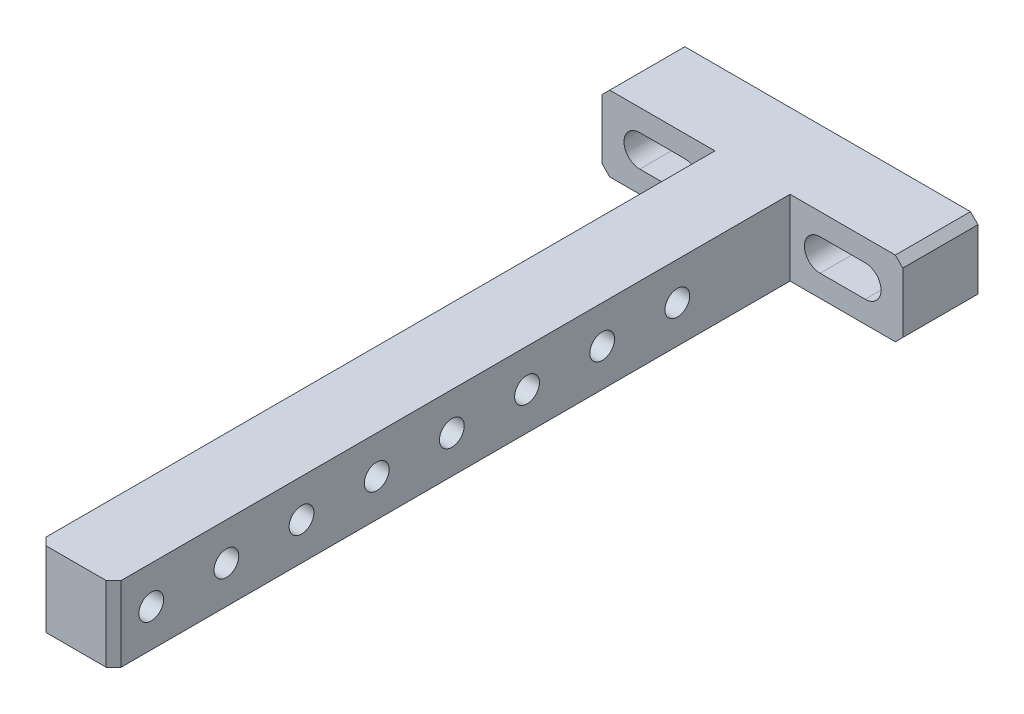
from build123d import *

# Parameters (mm, degrees)
SKETCH1_W           = 40
SKETCH1_H           = 10
BOSS_EXTRUDE1_DEPTH = 10
SKETCH2_W           = 10
SKETCH2_H           = 10
BOSS_EXTRUDE2_DEPTH = 90
CUT_EXTRUDE1_DEPTH  = 103.102889283
M4_TAPPED_HOLE1_D   = 3.3
CHAMFER1_SIZE       = 1


with BuildPart() as part:
    # Sketch1 → Boss-Extrude1 (new body)
    with BuildSketch(Plane.XY):
        Rectangle(SKETCH1_W, SKETCH1_H)
    extrude(amount=BOSS_EXTRUDE1_DEPTH)

    # Sketch2 → Boss-Extrude2 (add)
    with BuildSketch(Plane.XY.offset(10)):
        Rectangle(SKETCH2_W, SKETCH2_H)
    extrude(amount=BOSS_EXTRUDE2_DEPTH)

    # Sketch3 → Cut-Extrude1 (cut, through all)
    with BuildSketch(Plane(origin=(0, 0, 0), x_dir=(-1, 0, 0), z_dir=(0, 0, -1))):
        with BuildLine():
            Line((-15, 2.1), (-9, 2.1))
            ThreePointArc((-9, 2.1), (-6.9, 0), (-9, -2.1))
            Line((-9, -2.1), (-15, -2.1))
            ThreePointArc((-15, -2.1), (-17.1, 0), (-15, 2.1))
        make_face()
        with BuildLine():
            Line((15, 2.1), (9, 2.1))
            ThreePointArc((9, 2.1), (6.9, 0), (9, -2.1))
            Line((9, -2.1), (15, -2.1))
            ThreePointArc((15, -2.1), (17.1, 0), (15, 2.1))
        make_face()
    extrude(amount=-CUT_EXTRUDE1_DEPTH, mode=Mode.SUBTRACT)

    # M4 Tapped Hole1 (through all)
    with Locations(Plane(origin=(5, 0, 0), x_dir=(0, 0, -1), z_dir=(1, 0, 0))):
        with Locations((-25, 0), (-35, 0), (-45, 0), (-55, 0), (-65, 0), (-75, 0), (-85, 0), (-95, 0)):
            Hole(M4_TAPPED_HOLE1_D / 2)

    # Chamfer1
    chamfer1_edges = [part.edges().sort_by_distance(p)[0] for p in [
        (20, 5, 5),
        (20, -5, 5),
        (-20, -5, 5),
        (-20, 5, 5),
        (5, 0, 100),
        (-5, 0, 100),
    ]]
    chamfer(chamfer1_edges, length=CHAMFER1_SIZE)


solid = part.part
